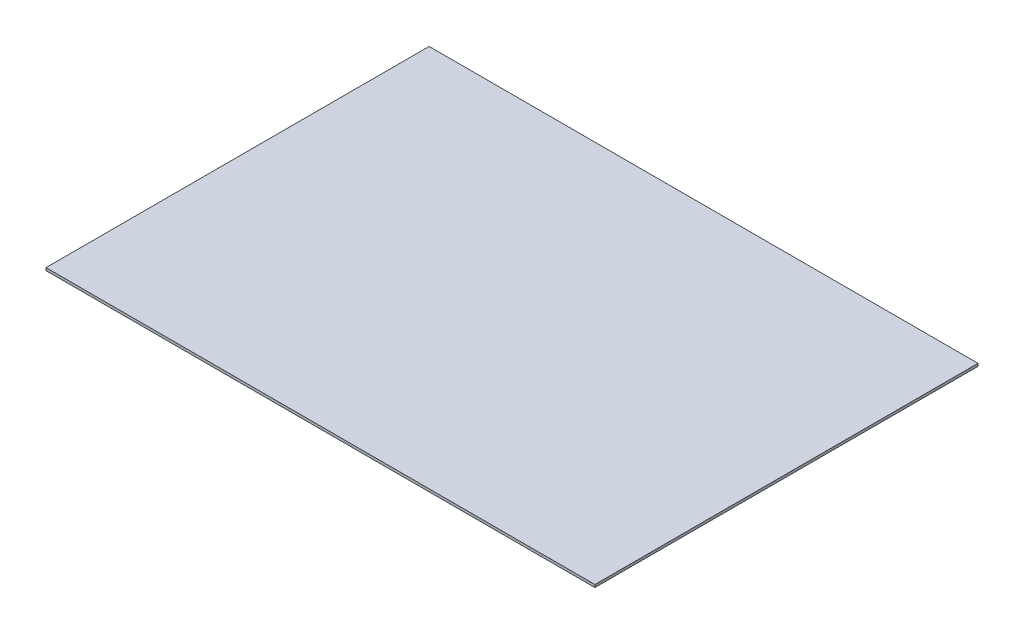
from build123d import *

# Parameters (mm, degrees)
SKETCH_1_W      = 415.5
SKETCH_1_H      = 290
EXTRUDE_1_DEPTH = 2


with BuildPart() as part:
    # 草图1 → 凸台-拉伸1 (new body)
    with BuildSketch(Plane(origin=(0, 0, 0), x_dir=(1, 0, 0), z_dir=(0, 1, 0))):
        Rectangle(SKETCH_1_W, SKETCH_1_H)
    extrude(amount=EXTRUDE_1_DEPTH)


solid = part.part
